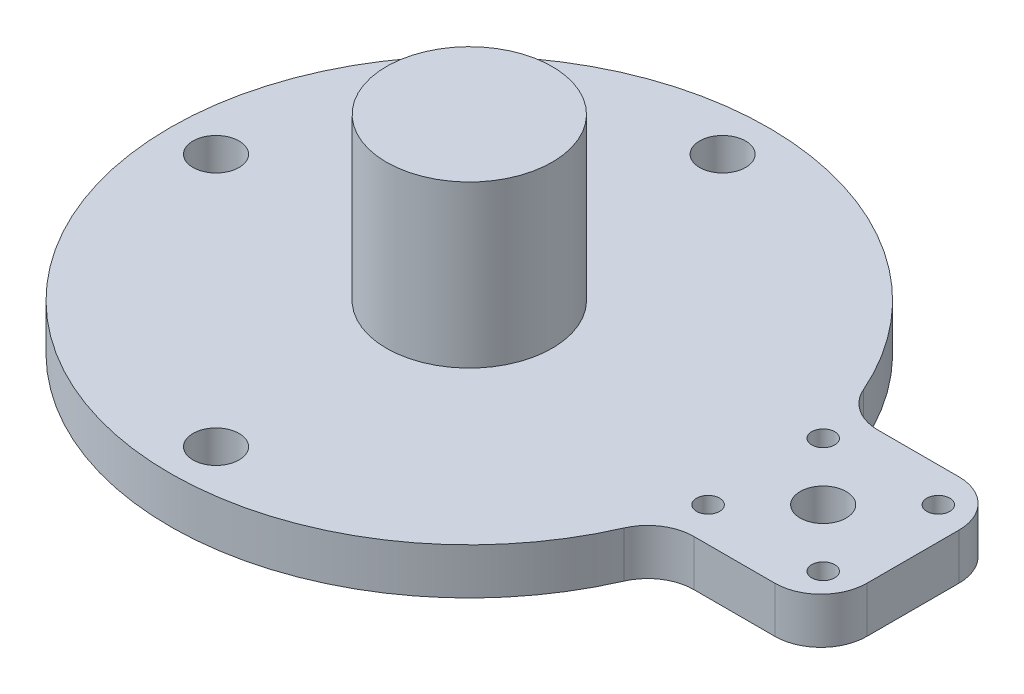
SolidWorks part; units mm, degrees
ref_plane "Front Plane" through (0, 0, 0) normal (0, 0, 1) x (1, 0, 0)
ref_plane "Top Plane" through (0, 0, 0) normal (0, 1, 0) x (1, 0, 0)
ref_plane "Right Plane" through (0, 0, 0) normal (1, 0, 0) x (0, 0, -1)
sketch "Sketch1" plane through (0, 0, 0) normal (0, 1, 0) x (1, 0, 0)
  circle A0 centre (0, 0) radius 450
  circle A1 centre (0, 0) radius 400
  dimension "D1" = 900
  dimension "D2" = 800
extrude "Boss-Extrude1" add sketch "Sketch1" along normal mid plane 1500
sketch "Sketch2" plane through (0, -750, 0) normal (0, -1, 0) x (1, 0, 0)
  circle A0 centre (0, 0) radius 650
  dimension "D1" = 1300
extrude "Boss-Extrude2" add sketch "Sketch2" along normal blind 100
sketch "Sketch3" plane through (0, -850, 0) normal (0, -1, 0) x (1, 0, 0)
  circle A0 centre (0, 0) radius 550 construction
  circle A1 centre (0, 550) radius 50
  circle A3 centre (550, 0) radius 50
  circle A4 centre (0, -550) radius 50
  circle A5 centre (-550, 0) radius 50
  point P14 (0, 0)
  dimension "D1" = 1100
  dimension "D2" = 100
  dimension "D3" = 4
extrude "Cut-Extrude1" cut sketch "Sketch3" against normal through all
sketch "Sketch4" plane through (0, -850, 0) normal (0, -1, 0) x (1, 0, 0)
  line L1 (-700, -1000) -> (700, -1000)
  line L2 (-1000, -700) -> (-1000, 700)
  line L3 (-700, 1000) -> (700, 1000)
  line L4 (1000, -700) -> (1000, 700)
  line L5 (-1000, -1000) -> (1000, 1000) construction
  line L6 (-1000, 1000) -> (1000, -1000) construction
  arc A0 (-1000, 700) -> (-700, 1000) centre (-700, 700) cw
  arc A1 (700, 1000) -> (1000, 700) centre (700, 700) cw
  arc A2 (700, -1000) -> (1000, -700) centre (700, -700) ccw
  arc A3 (-700, -1000) -> (-1000, -700) centre (-700, -700) cw
  circle A4 centre (-700, -700) radius 100
  circle A5 centre (700, -700) radius 100
  circle A6 centre (700, 700) radius 100
  circle A7 centre (-700, 700) radius 100
  point P0 (0, 0)
  dimension "D3" = 300
  dimension "D4" = 200
  dimension "D5" = 200
  dimension "D6" = 200
  dimension "D7" = 200
  dimension "D1" = 2000
  dimension "D2" = 2000
extrude "Boss-Extrude3" add sketch "Sketch4" along normal blind 200
mirror "Mirror1" about plane through (0, 0, 0) normal (0, 1, 0) of "Cut-Extrude1", "Boss-Extrude2"
sketch "Sketch6" plane through (0, 850, 0) normal (0, 1, 0) x (1, 0, 0)
  circle A0 centre (0, 0) radius 400
  dimension "D1" = 800
extrude "Cut-Extrude2" cut sketch "Sketch6" against normal blind 200
sketch "Sketch7" plane through (0, -750, 0) normal (0, 1, 0) x (1, 0, 0)
  circle A0 centre (0, 0) radius 400
extrude "Boss-Extrude4" add sketch "Sketch7" along normal up to surface (1600 mm away)
sketch "Sketch8" plane through (0, 850, 0) normal (0, 1, 0) x (1, 0, 0)
  circle A0 centre (0, 0) radius 180
  dimension "D1" = 360
extrude "Boss-Extrude5" add sketch "Sketch8" along normal blind 350
sketch "Sketch9" plane through (0, 850, 0) normal (0, 1, 0) x (1, 0, 0)
  line L1 (618.4658, 200) -> (963.4658, 200)
  line L2 (618.4658, 200) -> (618.4658, -78.9961)
  line L3 (618.4658, -200) -> (963.4658, -200)
  line L4 (963.4658, 200) -> (963.4658, -200)
  line L5 (618.4658, -78.9961) -> (618.4658, -200)
  circle A0 centre (0, 0) radius 650 construction
  circle A1 centre (550, 0) radius 50
  circle A2 centre (0, 0) radius 650 construction
  dimension "D1" = 345
  dimension "D2" = 200
extrude "Boss-Extrude6" add sketch "Sketch9" against normal up to surface (100 mm away)
sketch "Sketch10" plane through (0, 850, 0) normal (0, 1, 0) x (1, 0, 0)
  line L0 (963.4658, -200) -> (963.4658, 200) construction
  line L1 (643.4658, -125) -> (893.4658, -125) construction
  line L2 (643.4658, -125) -> (643.4658, 125) construction
  line L3 (643.4658, 125) -> (893.4658, 125) construction
  line L4 (893.4658, -125) -> (893.4658, 125) construction
  line L5 (643.4658, -125) -> (893.4658, 125) construction
  line L6 (643.4658, 125) -> (893.4658, -125) construction
  line L7 (618.4658, -200) -> (963.4658, -200) construction
  circle A0 centre (893.4658, 125) radius 25
  circle A1 centre (643.4658, 125) radius 25
  circle A2 centre (643.4658, -125) radius 25
  circle A3 centre (893.4658, -125) radius 25
  circle A4 centre (768.4658, 0) radius 50
  point P0 (768.4658, 0)
  dimension "D5" = 50
  dimension "D6" = 50
  dimension "D7" = 50
  dimension "D8" = 50
  dimension "D9" = 100
  dimension "D1" = 250
  dimension "D2" = 250
  dimension "D3" = 70
  dimension "D4" = 75
extrude "Cut-Extrude3" cut sketch "Sketch10" against normal up to next
fillet "Fillet1" radius 100 4 edges at (618.4658, 800, -200) (618.4658, 800, 200) (963.4658, 800, 200) (963.4658, 800, -200)
sketch "Sketch11" plane through (0, -1050, 0) normal (0, -1, 0) x (1, 0, 0)
  circle A0 centre (0, 0) radius 2346.179
extrude "Cut-Extrude4" cut sketch "Sketch11" against normal up to surface (1800 mm away)
